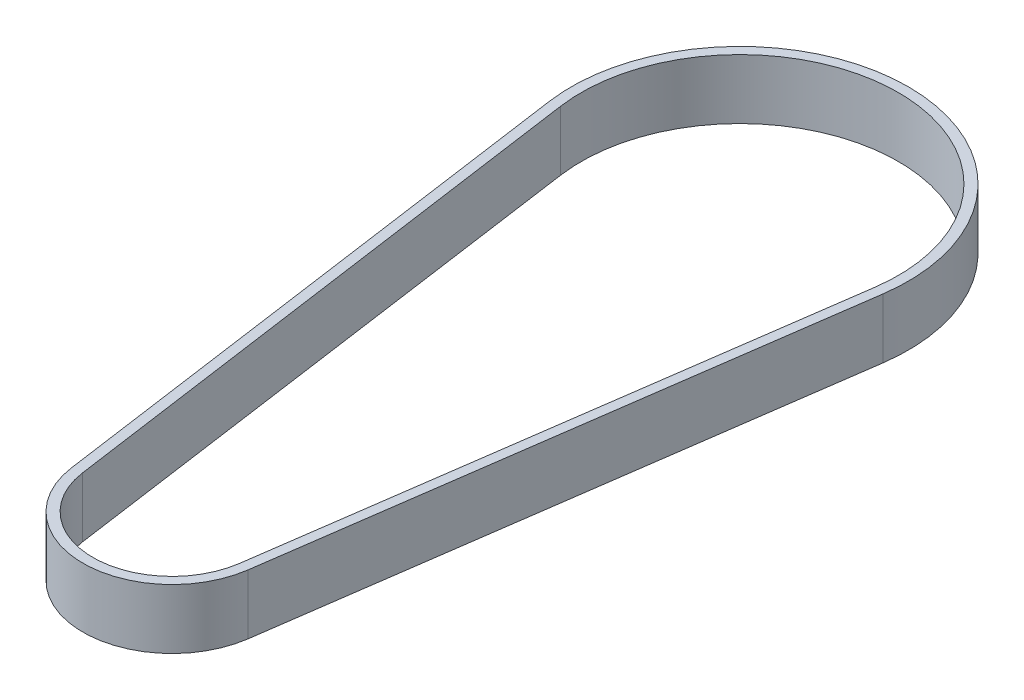
SolidWorks part; units mm, degrees
ref_plane "Front Plane" through (0, 0, 0) normal (0, 0, 1) x (1, 0, 0)
ref_plane "Top Plane" through (0, 0, 0) normal (0, 1, 0) x (1, 0, 0)
ref_plane "Right Plane" through (0, 0, 0) normal (1, 0, 0) x (0, 0, -1)
sketch "Sketch1" plane through (0, 0, 0) normal (0, 1, 0) x (1, 0, 0)
  line L0 (0, 0) -> (0, 57) construction
  line L1 (-15.7581, 54.7776) -> (-7.8761, -1.1108)
  line L2 (15.7581, 54.7776) -> (7.8761, -1.1108)
  line L3 (-16.7483, 54.638) -> (-8.8663, -1.2504)
  line L4 (16.7483, 54.638) -> (8.8663, -1.2504)
  arc A0 (-7.8761, -1.1108) -> (7.8761, -1.1108) centre (0, 0) ccw
  arc A1 (15.7581, 54.7776) -> (-15.7581, 54.7776) centre (0, 57) ccw
  arc A2 (-8.8663, -1.2504) -> (8.8663, -1.2504) centre (0, 0) ccw
  arc A3 (16.7483, 54.638) -> (-16.7483, 54.638) centre (0, 57) ccw
  dimension "D1" = 7.954
  dimension "D2" = 15.914
  dimension "D3" = 57
  dimension "D4" = 1
extrude "Boss-Extrude1" add sketch "Sketch1" along normal blind 6
